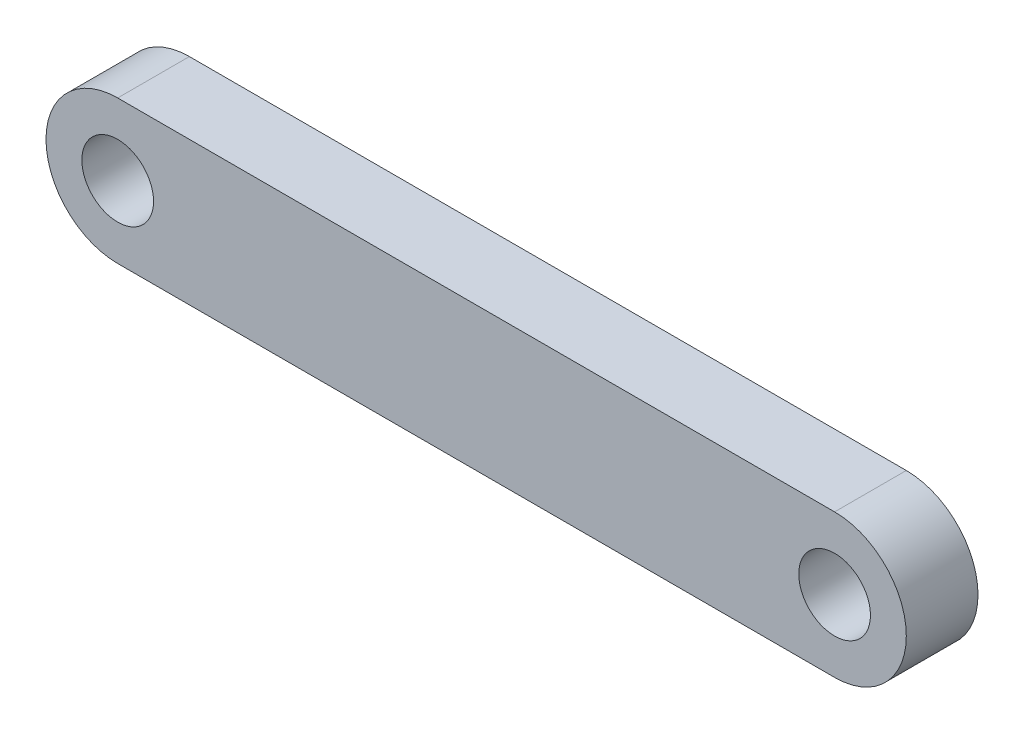
SolidWorks part; units mm, degrees
material "普通碳钢"
ref_plane "Front Plane" through (0, 0, 0) normal (0, 0, 1) x (1, 0, 0)
ref_plane "Top Plane" through (0, 0, 0) normal (0, 1, 0) x (1, 0, 0)
ref_plane "Right Plane" through (0, 0, 0) normal (1, 0, 0) x (0, 0, -1)
sketch "Sketch1" plane through (0, 0, 0) normal (0, 0, 1) x (1, 0, 0)
  line L1 (-25, 10) -> (75, 10)
  line L3 (-25, -10) -> (75, -10)
  arc A0 (-25, 10) -> (-25, -10) centre (-25, 0) ccw
  arc A1 (75, -10) -> (75, 10) centre (75, 0) ccw
  circle A2 centre (75, 0) radius 5
  circle A3 centre (-25, 0) radius 5
  point P0 (0, 0)
  dimension "D3" = 10
  dimension "D1" = 100
  dimension "D2" = 20
extrude "Boss-Extrude1" add sketch "Sketch1" along normal blind 10
